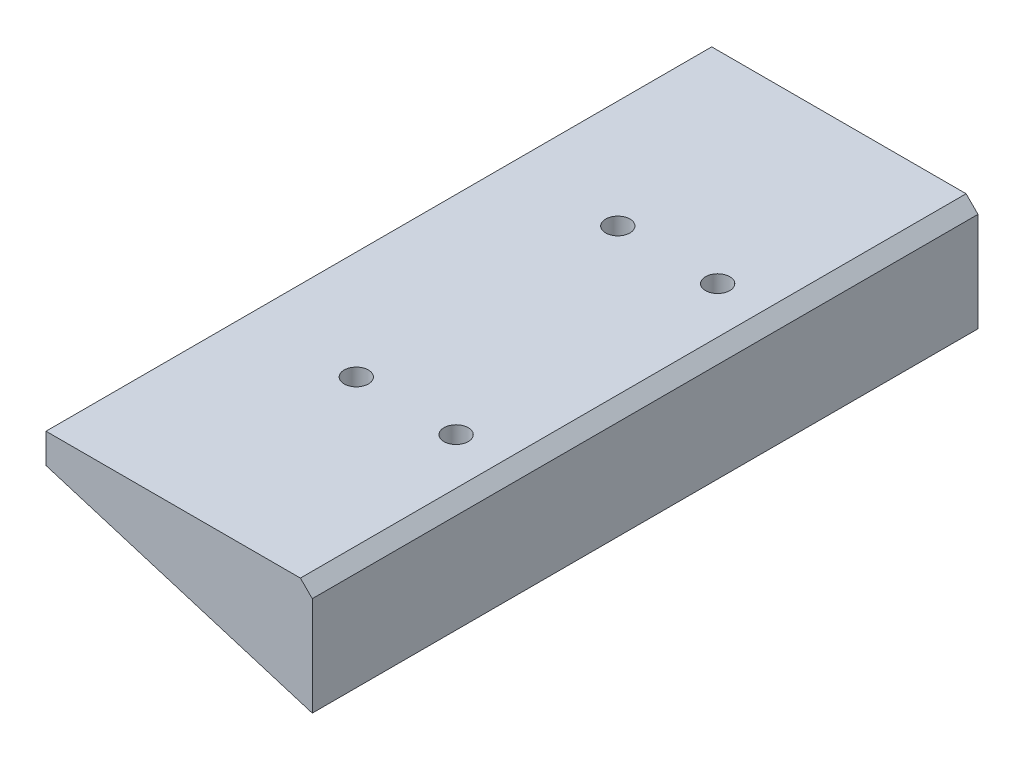
SolidWorks part; units mm, degrees
ref_plane "Front Plane" through (0, 0, 0) normal (0, 0, 1) x (1, 0, 0)
ref_plane "Top Plane" through (0, 0, 0) normal (0, 1, 0) x (1, 0, 0)
ref_plane "Right Plane" through (0, 0, 0) normal (1, 0, 0) x (0, 0, -1)
sketch "Sketch1" plane through (0, 0, 0) normal (0, 0, 1) x (1, 0, 0)
  line L0 (0, 0) -> (0, 12.5)
  line L1 (0, 12.5) -> (107, 12.5)
  line L2 (112, 7.5) -> (112, -34.2)
  line L3 (112, -34.2) -> (0, 0)
  line L4 (107, 12.5) -> (112, 7.5)
  point P4 (112, 12.5)
  dimension "D1" = 12.5
  dimension "D2" = 112
  dimension "D3" = 46.7
extrude "Boss-Extrude1" add sketch "Sketch1" along normal blind 280
hole_wizard "M12 Tapped Hole1" positions "Sketch3" profile "Sketch2" tap size "M12" standard "GB" end condition through all
sketch "Sketch3" plane through (0, 12.5, 0) normal (0, 1, 0) x (-1, 0, 0)
  line L0 (-45.5, 26.5066) -> (-45.5, 219.5943) construction
  line L1 (-87.5, 30.6317) -> (-87.5, 228.0593) construction
  line L2 (-12.5995, 85) -> (-102.4084, 85) construction
  line L3 (-12.5995, 195) -> (-102.4084, 195) construction
  line L4 (0, 280) -> (0, 0) construction
  line L5 (-107, 0) -> (0, 0) construction
  point P0 (-45.5, 195)
  point P1 (-45.5, 85)
  point P3 (-87.5, 85)
  point P5 (-87.5, 195)
  dimension "D1" = 45.5
  dimension "D2" = 42
  dimension "D3" = 85
  dimension "D4" = 110
sketch "Sketch2" plane through (45.5, 12.5, 195) normal (1, 0, 0) x (0, 0, 1)
  line L0 (0, 0) -> (0, 46.7)
  line L1 (0, 46.7) -> (5.1, 46.7)
  line L2 (5.1, 46.7) -> (5.1, 0)
  line L5 (5.1, 0) -> (0, 0)
  line L11 (0, -6.35) -> (0, 107.95) construction
  dimension "通孔螺纹孔钻头直径" = 10.2
  dimension "通孔螺纹孔钻头深度" = 46.7
cosmetic thread "Cosmetic Thread 1" parameters "D2"=12
cosmetic thread "Cosmetic Thread 2" parameters "D2"=12
cosmetic thread "Cosmetic Thread 3" parameters "D2"=12
cosmetic thread "Cosmetic Thread 4" parameters "D2"=12
